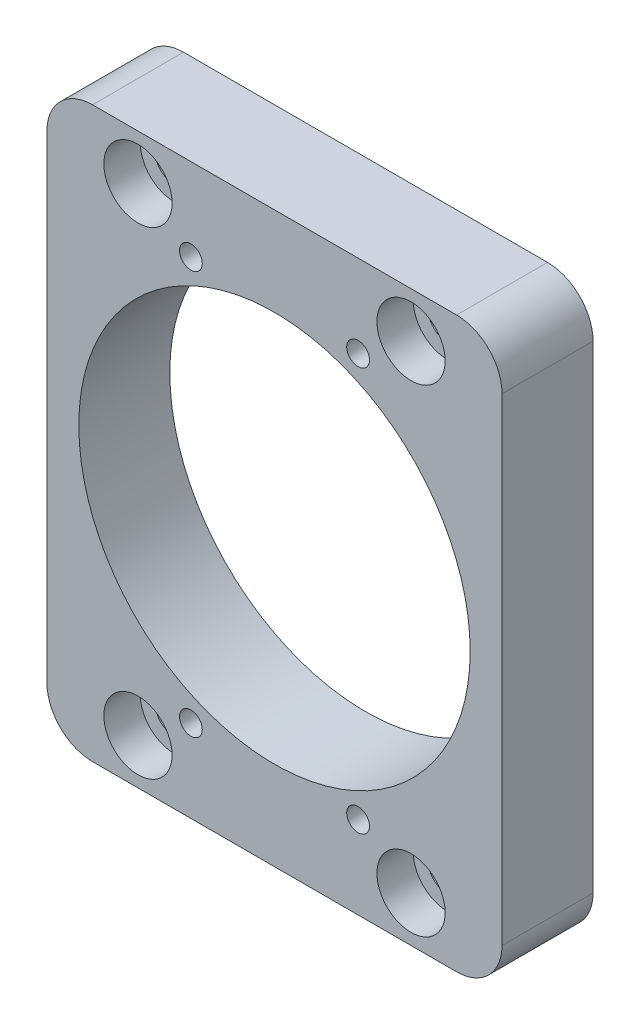
from build123d import *

# Parameters (mm, degrees)
SKETCH_1_W                   = 100
SKETCH_1_H                   = 125
EXTRUDE_1_DEPTH              = 20
HOLE_WIZARD_M8_1_D           = 8.5
HOLE_WIZARD_M8_1_CBORE_D     = 15
HOLE_WIZARD_M8_1_CBORE_DEPTH = 8
SKETCH_4_R                   = 43
CUT_EXTRUDE_1_DEPTH          = 83.5
HOLE_WIZARD_M6_1_D           = 5
FILLET_1_R                   = 10


with BuildPart() as part:
    # 草图1 → 凸台-拉伸1 (new body)
    with BuildSketch(Plane.XY):
        Rectangle(SKETCH_1_W, SKETCH_1_H)
    extrude(amount=EXTRUDE_1_DEPTH)

    # M8 六角凹头螺钉的柱形沉头孔1 (through all)
    with Locations(Plane.XY.offset(20)):
        with Locations((-30, -52.5), (30, -52.5)):
            hole_wizard_m8_1 = CounterBoreHole(HOLE_WIZARD_M8_1_D / 2, HOLE_WIZARD_M8_1_CBORE_D / 2, HOLE_WIZARD_M8_1_CBORE_DEPTH)

    # 草图4 → 切除-拉伸1 (cut, through all)
    with BuildSketch(Plane.XY.offset(20)):
        Circle(SKETCH_4_R)
    extrude(amount=-CUT_EXTRUDE_1_DEPTH, mode=Mode.SUBTRACT)

    # M6 螺纹孔1 (through all)
    with Locations(Plane.XY.offset(20)):
        with Locations((-18.368804754, 44.346217561), (18.368804754, 44.346217561)):
            hole_wizard_m6_1 = Hole(HOLE_WIZARD_M6_1_D / 2)

    # 镜向2: M8 六角凹头螺钉的柱形沉头孔1, M6 螺纹孔1 across plane
    add(hole_wizard_m8_1.mirror(Plane.ZX), mode=Mode.SUBTRACT)
    add(hole_wizard_m6_1.mirror(Plane.ZX), mode=Mode.SUBTRACT)

    # 圆角1
    fillet_1_edges = [part.edges().sort_by_distance(p)[0] for p in [
        (-50, 62.5, 10),
        (50, 62.5, 10),
        (50, -62.5, 10),
        (-50, -62.5, 10),
    ]]
    fillet(fillet_1_edges, radius=FILLET_1_R)


solid = part.part
